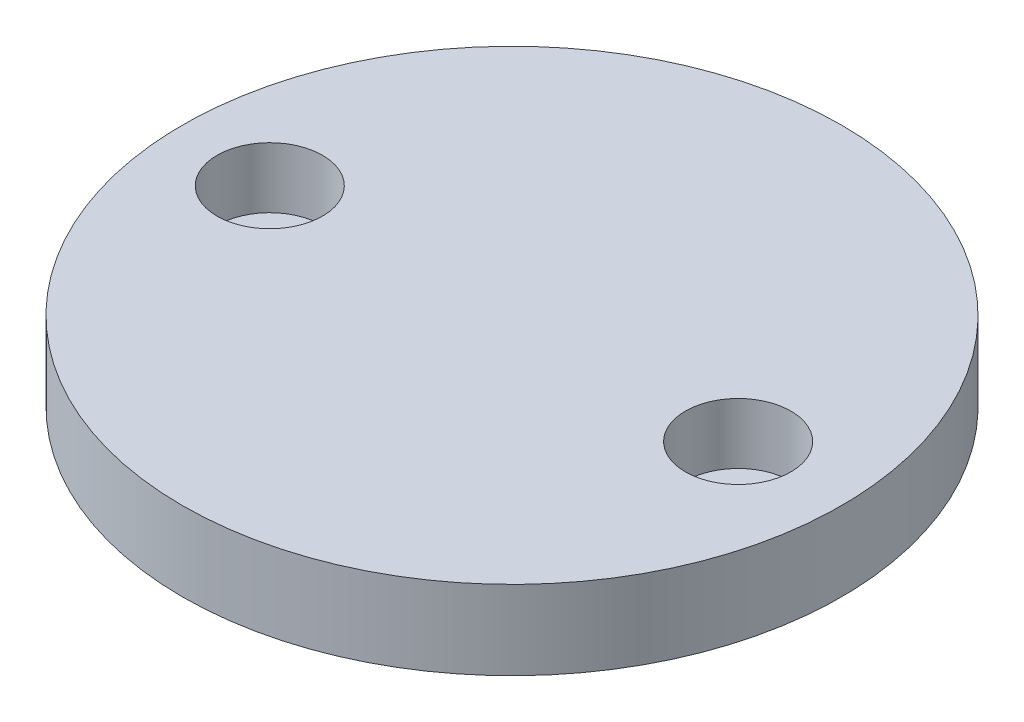
from build123d import *

# Parameters (mm, degrees)
SKETCH1_R                                            = 25
BOSS_EXTRUDE1_DEPTH                                  = 6
HOLE_SIZE_BASED_ON_SOCKET_HEAD_CAP_SCREW_D           = 4.5
HOLE_SIZE_BASED_ON_SOCKET_HEAD_CAP_SCREW_DEPTH       = 10.1
HOLE_SIZE_BASED_ON_SOCKET_HEAD_CAP_SCREW_CBORE_D     = 8
HOLE_SIZE_BASED_ON_SOCKET_HEAD_CAP_SCREW_CBORE_DEPTH = 4.6
HOLE_SIZE_BASED_ON_SOCKET_HEAD_CAP_SCREW_TIP         = 1.351936393


with BuildPart() as part:
    # Sketch1 → Boss-Extrude1 (new body)
    with BuildSketch(Plane(origin=(0, 0, 0), x_dir=(1, 0, 0), z_dir=(0, 1, 0))):
        with Locations(Location((0, 0, 0), (0, 0, 270))):
            Circle(SKETCH1_R)
    extrude(amount=BOSS_EXTRUDE1_DEPTH)

    # Hole size based on socket head cap screw type 1
    with Locations(Plane(origin=(16.864722122, 6, -0.289543132), x_dir=(0, 0, 1), z_dir=(0, 1, 0))):
        with Locations((0, 0), (0.961754182, -34.5679876)):
            CounterBoreHole(HOLE_SIZE_BASED_ON_SOCKET_HEAD_CAP_SCREW_D / 2, HOLE_SIZE_BASED_ON_SOCKET_HEAD_CAP_SCREW_CBORE_D / 2, HOLE_SIZE_BASED_ON_SOCKET_HEAD_CAP_SCREW_CBORE_DEPTH, depth=HOLE_SIZE_BASED_ON_SOCKET_HEAD_CAP_SCREW_DEPTH)
            with Locations((0, 0, -(HOLE_SIZE_BASED_ON_SOCKET_HEAD_CAP_SCREW_DEPTH + HOLE_SIZE_BASED_ON_SOCKET_HEAD_CAP_SCREW_TIP / 2))):  # 118° drill point
                Cone(0, HOLE_SIZE_BASED_ON_SOCKET_HEAD_CAP_SCREW_D / 2, HOLE_SIZE_BASED_ON_SOCKET_HEAD_CAP_SCREW_TIP, mode=Mode.SUBTRACT)


solid = part.part
